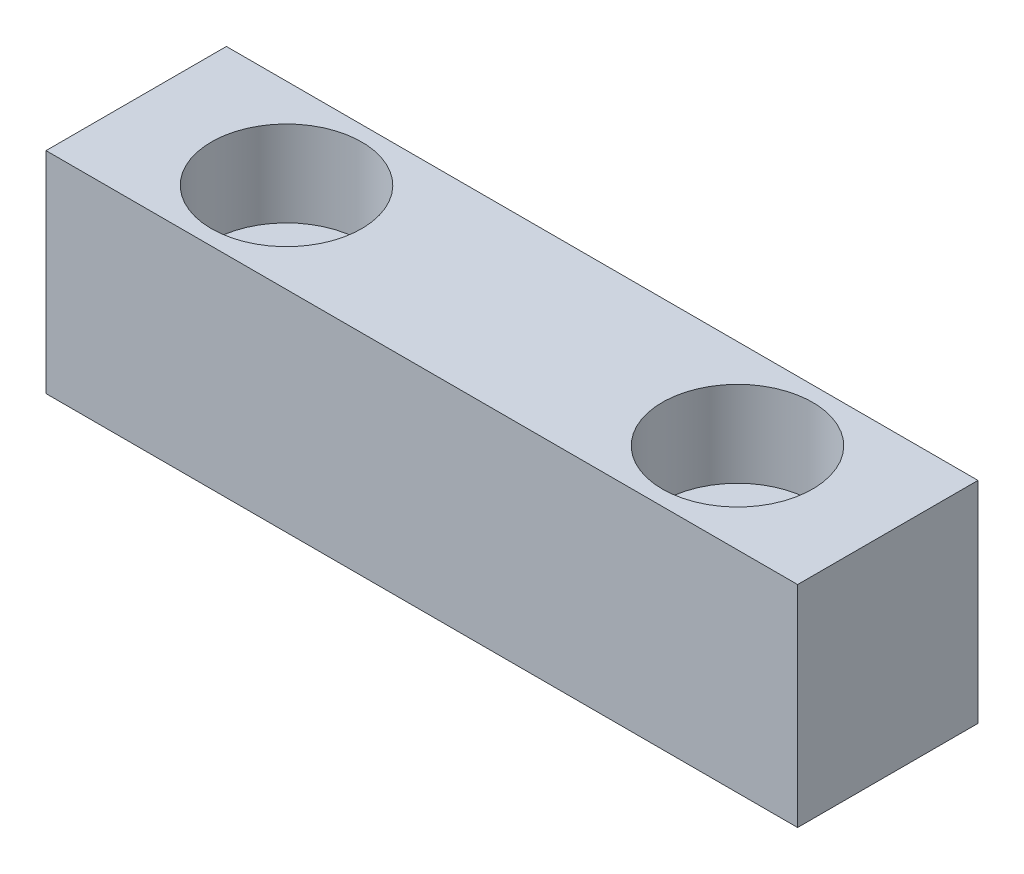
SolidWorks part; units mm, degrees
material "AL6061"
ref_plane "Front Plane" through (0, 0, 0) normal (0, 0, 1) x (1, 0, 0)
ref_plane "Top Plane" through (0, 0, 0) normal (0, 1, 0) x (1, 0, 0)
ref_plane "Right Plane" through (0, 0, 0) normal (1, 0, 0) x (0, 0, -1)
sketch "Sketch1" plane through (0, 0, 0) normal (0, 1, 0) x (1, 0, 0)
  line L9 (-25, -6) -> (25, -6)
  line L10 (-25, -6) -> (-25, 6)
  line L11 (-25, 6) -> (25, 6)
  line L12 (25, -6) -> (25, 6)
  line L13 (-25, -6) -> (25, 6) construction
  line L14 (-25, 6) -> (25, -6) construction
  point P0 (0, 0)
  dimension "D1" = 12
  dimension "D2" = 50
extrude "Boss-Extrude1" add sketch "Sketch1" along normal mid plane 14
hole_wizard "Hole Size (per socket head cap screw type)1" positions "Sketch2" profile "Sketch3" counterbore size "M5" standard "GB" end condition through all
sketch "Sketch2" plane through (0, 7, 0) normal (0, 1, 0) x (1, 0, 0)
  line L0 (0, 0) -> (0, 13.3258) construction
  line L3 (0, 0) -> (-32.8771, 0) construction
  line L4 (-25, 6) -> (-25, -6) construction
  point P13 (-15, 0)
  point P16 (15, 0)
  dimension "D1" = 10
sketch "Sketch3" plane through (15, 7, 0) normal (1, 0, 0) x (0, 0, 1)
  line L0 (0, 0) -> (0, 14)
  line L1 (0, 14) -> (2.75, 14)
  line L3 (2.75, 14) -> (2.75, 5.7)
  line L4 (2.75, 5.7) -> (5, 5.7)
  line L5 (5, 5.7) -> (5, 0)
  line L7 (5, 0) -> (0, 0)
  line L11 (0, -6.35) -> (0, 107.95) construction
  dimension "通孔孔直径" = 5.5
  dimension "通孔孔深度" = 14
  dimension "柱形沉头孔直径" = 10
  dimension "柱形沉头孔深度" = 5.7
